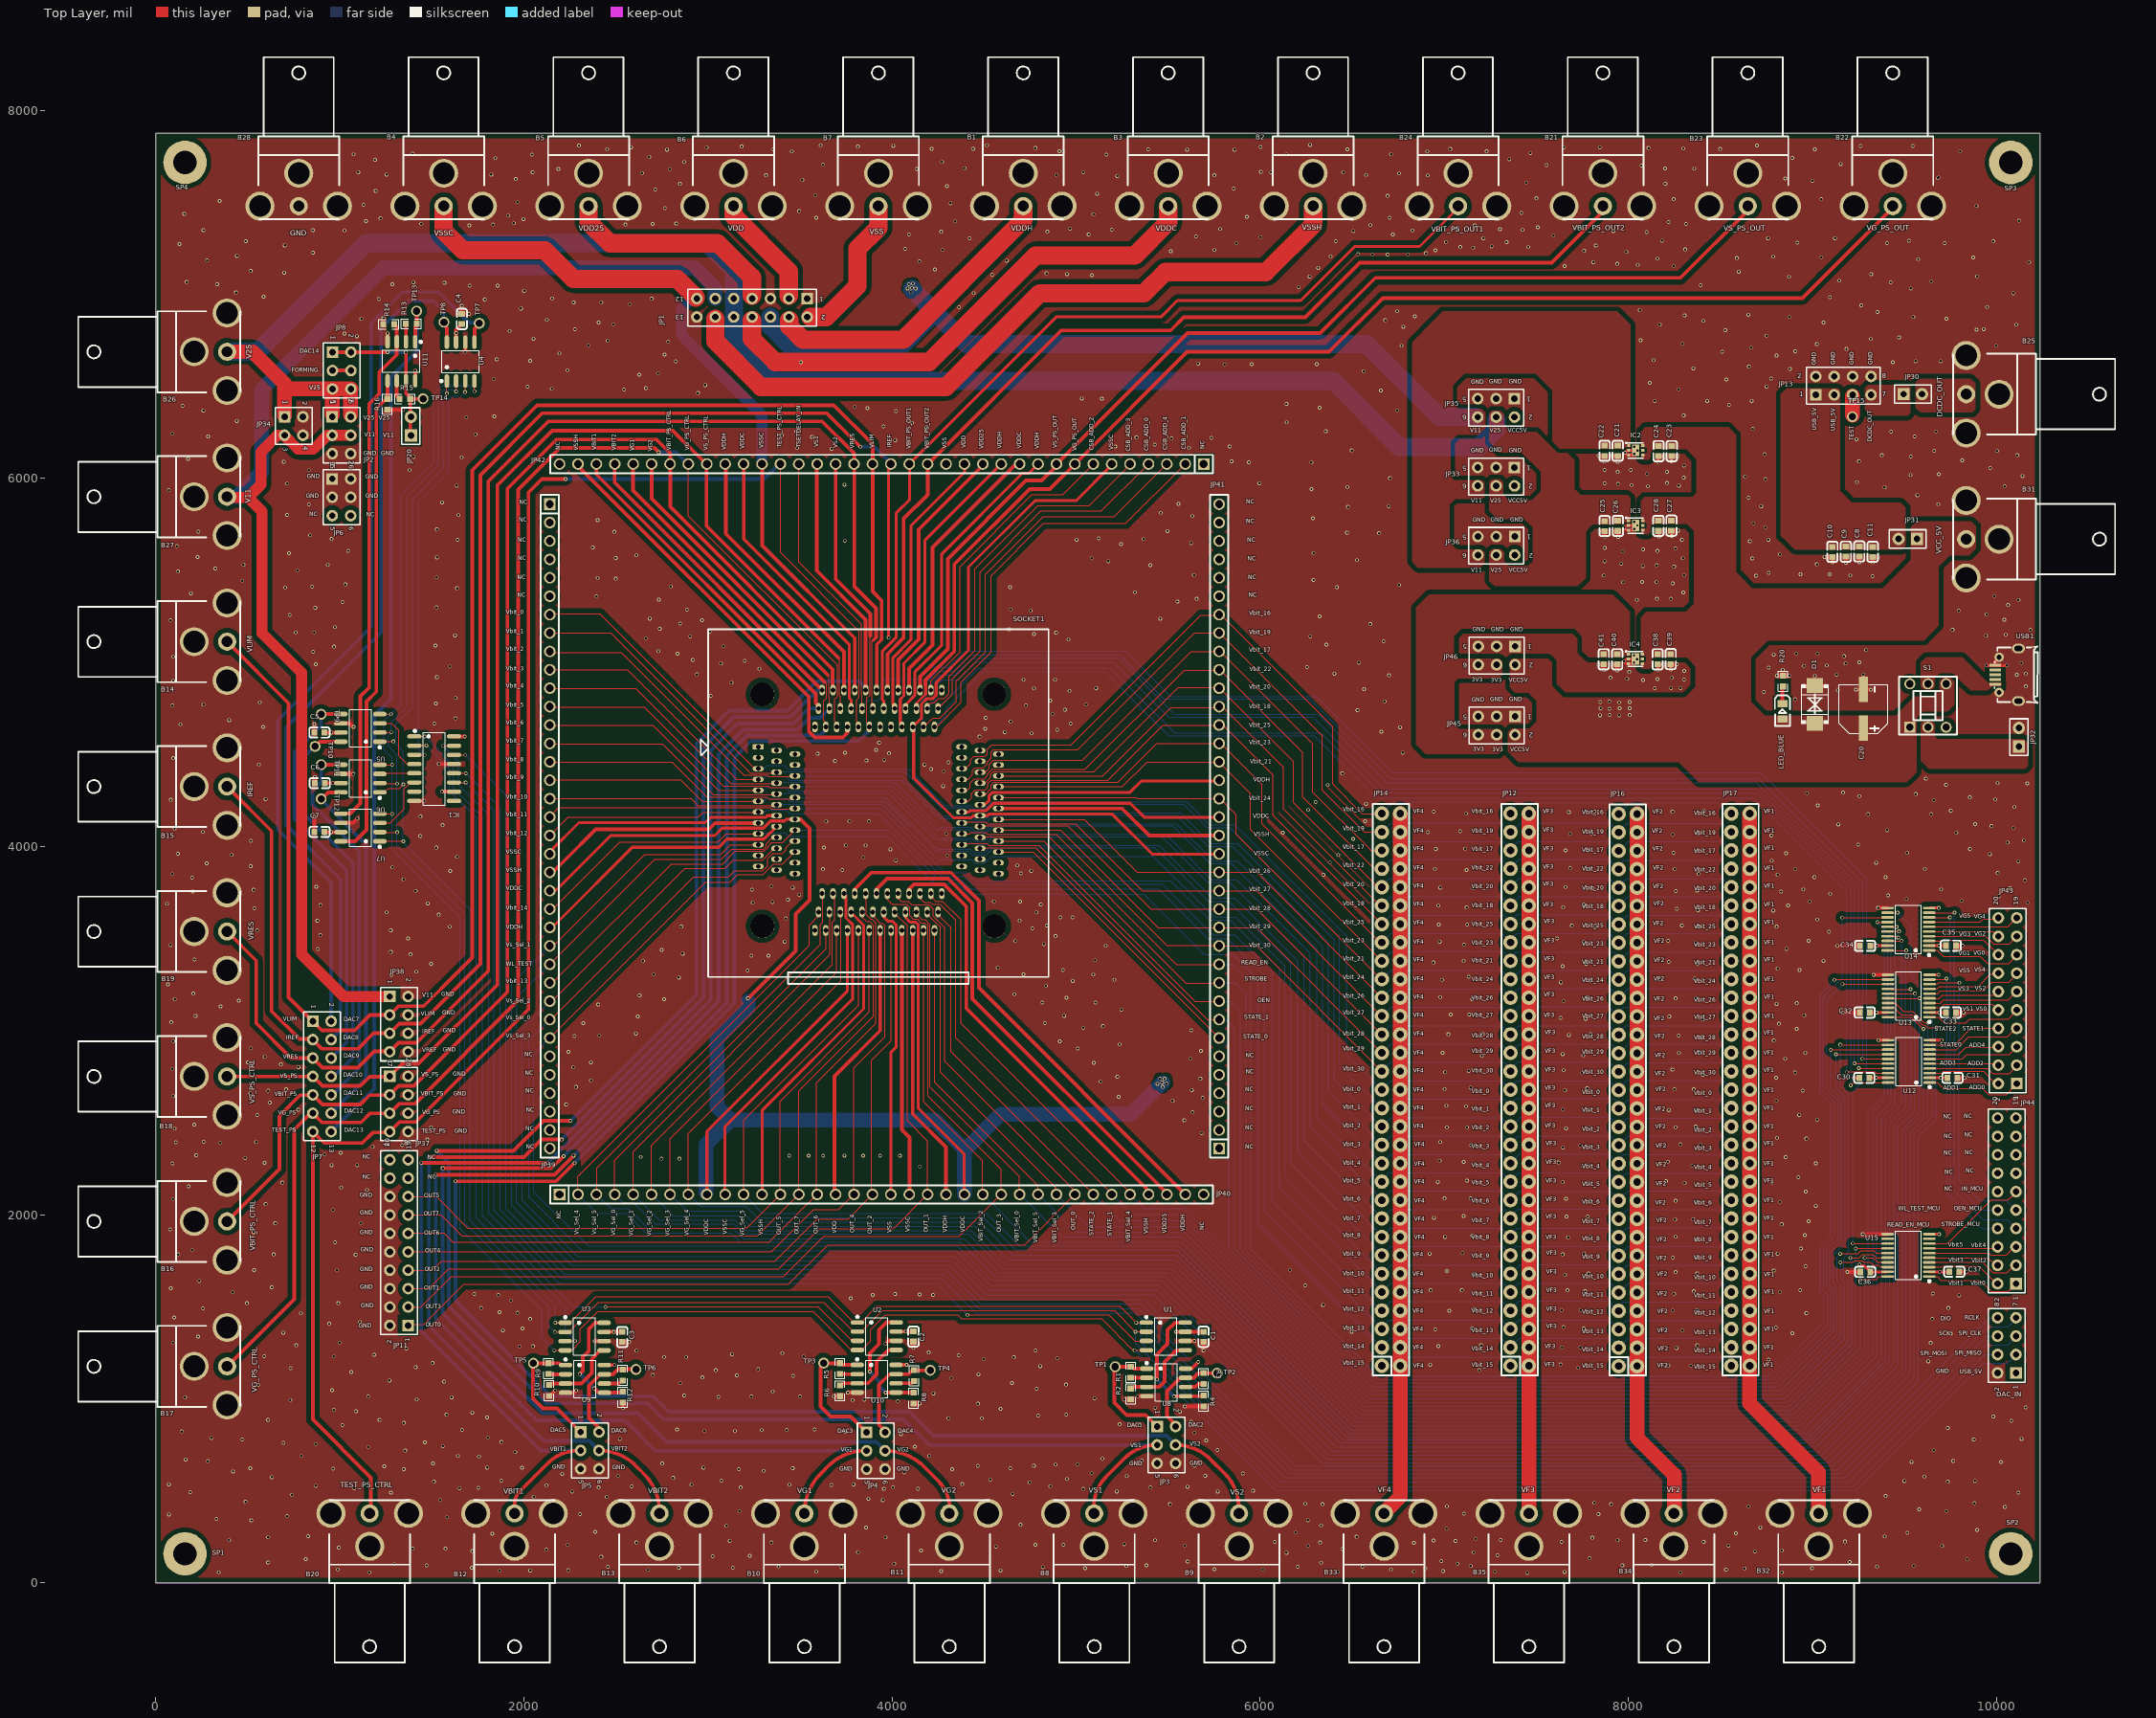
[diagram p0: Top Layer view]
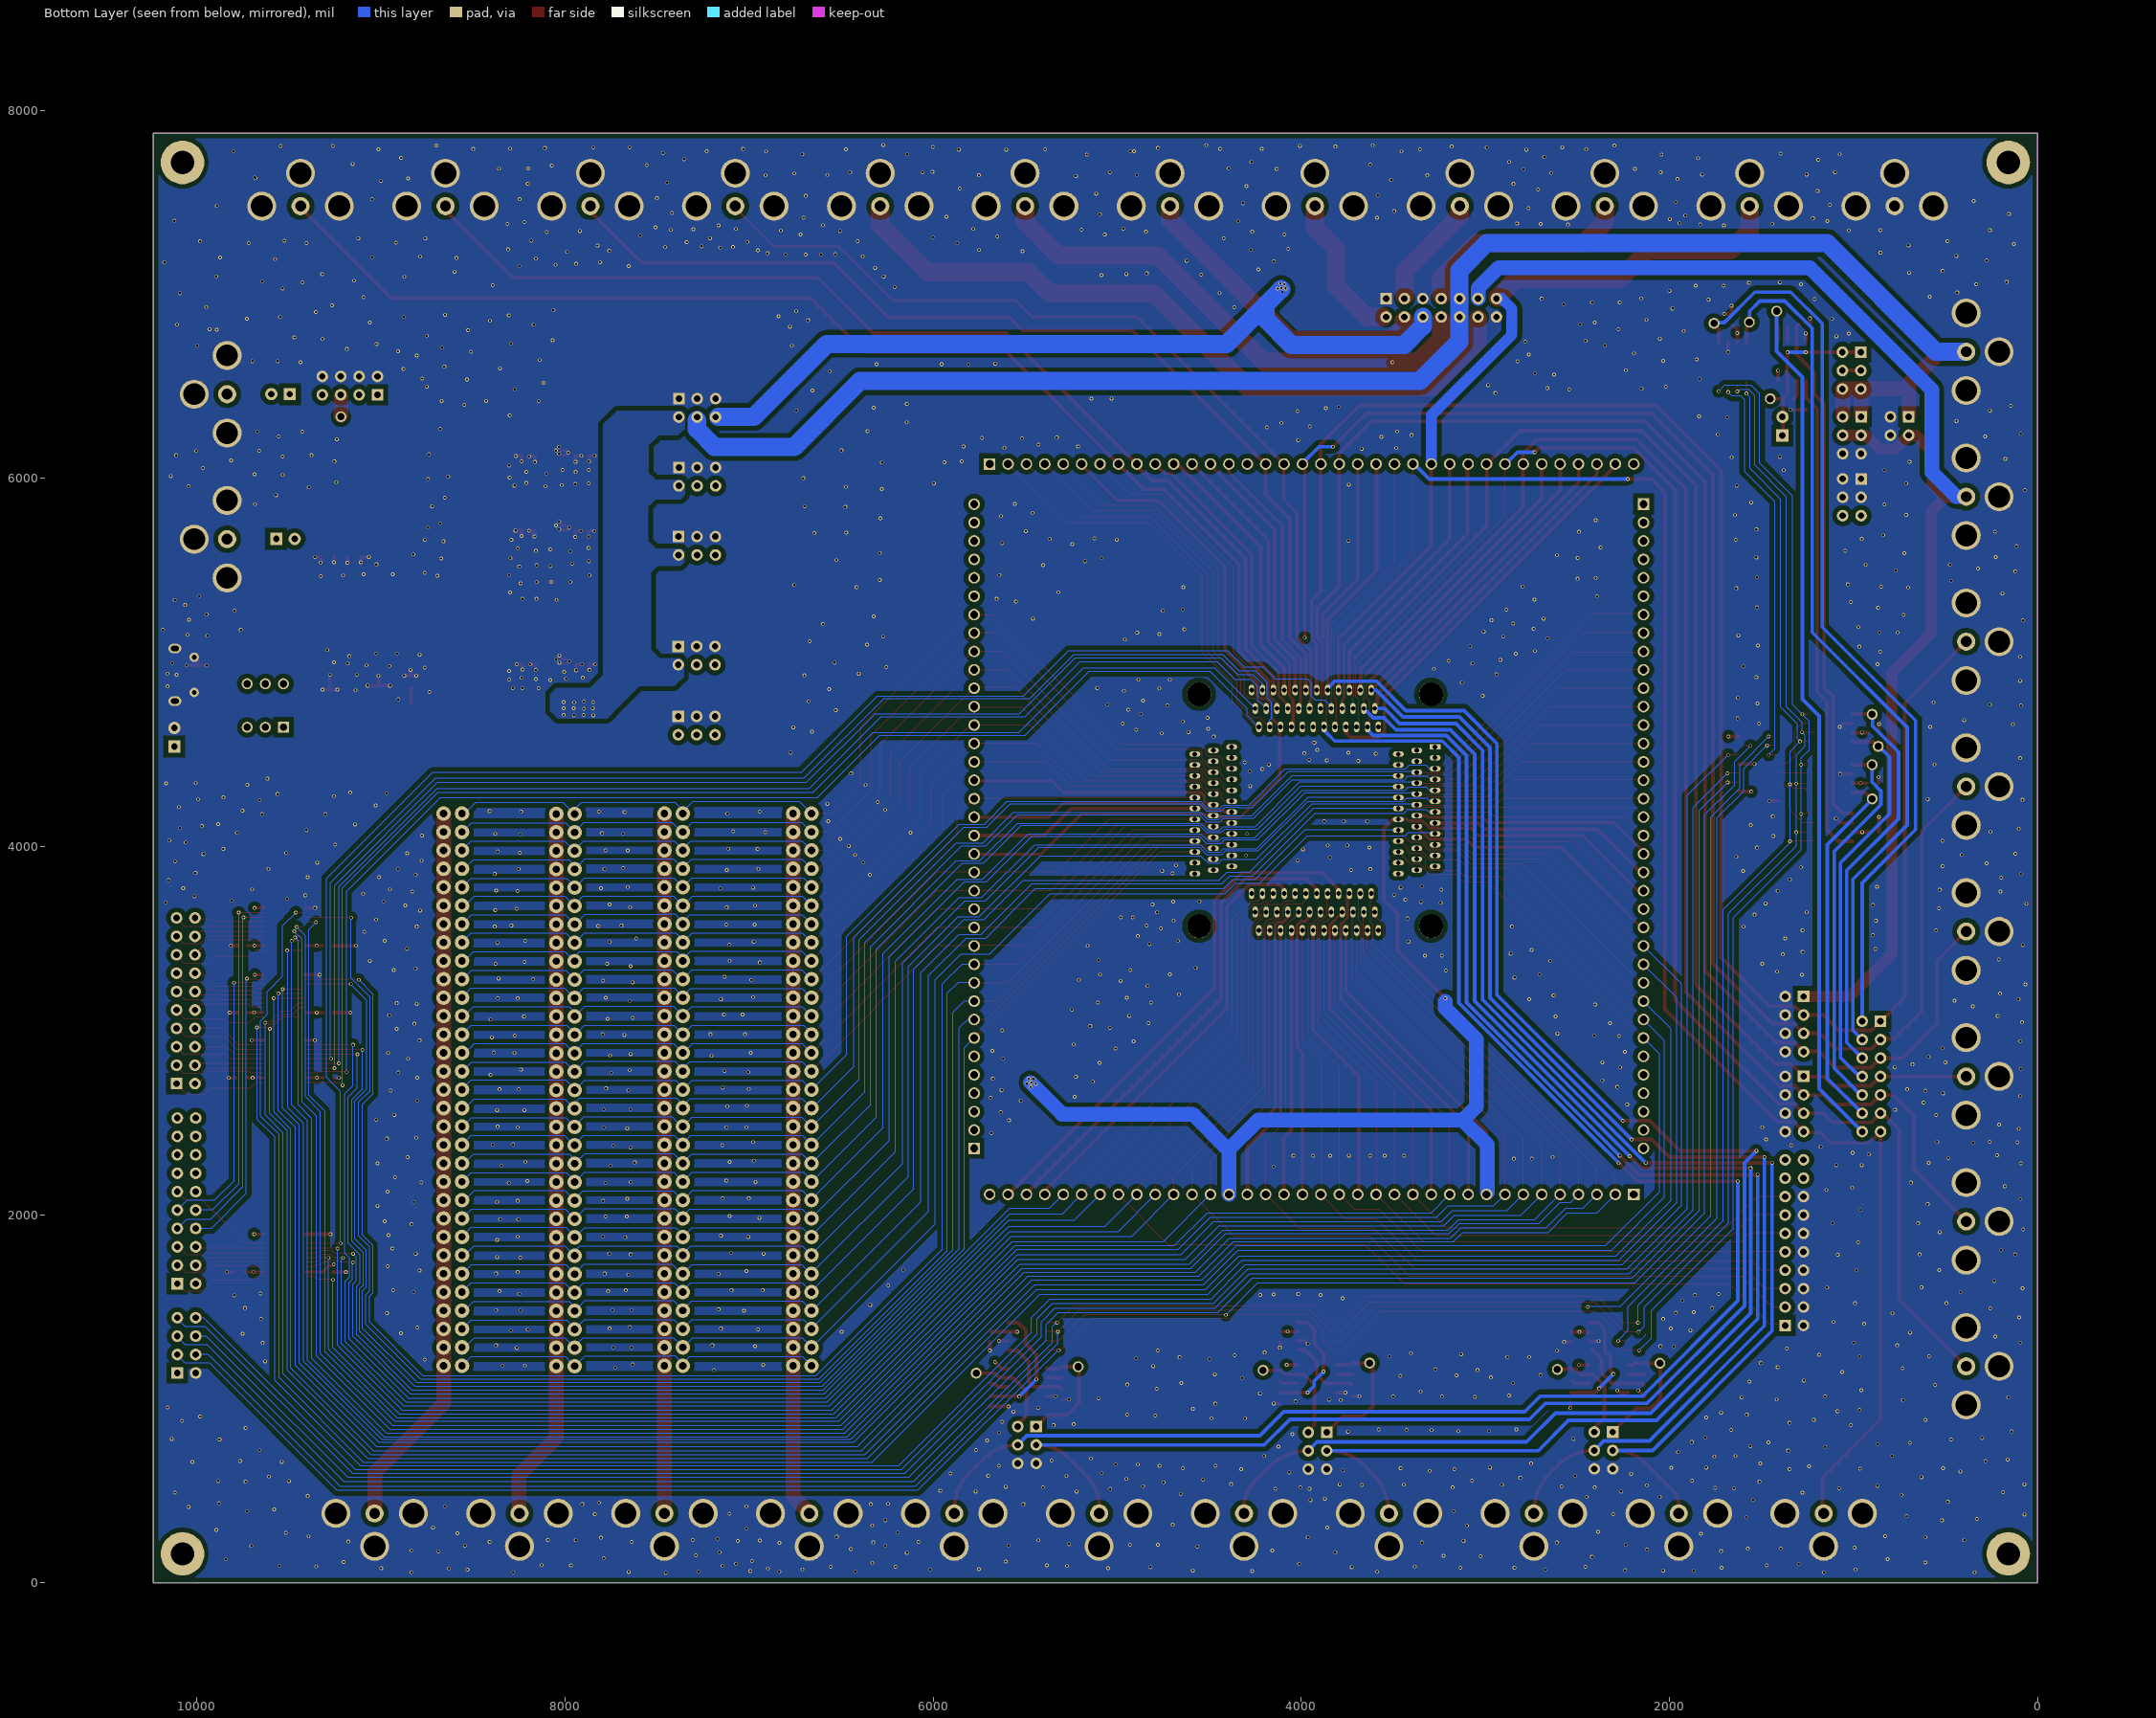
[diagram p1: Bottom Layer view, seen from below]
# Altium PCB MISC62794.PcbDoc (part 1 of 7)
Units mil, origin at the board's own origin, x right, y up, seen from the top; angles counter-clockwise.
Board outline 10236.22 x 7874.02 mil, 4 copper layers (Top Layer, GND, POWER, Bottom Layer); 158 components, 185 nets, 1211 pads, 1759 vias.

## Layer stack, top to bottom (the 12.6 mil dielectric is the usual default, probably not edited)
Top Layer: signal copper 1.4
Dielectric: core 12.6, FR-4, Dk 4.8
GND: plane copper 1.4, net GND
Dielectric: prepreg 12.6, FR-4, Dk 4.8
POWER: signal copper 1.4
Dielectric: core 12.6, FR-4, Dk 4.8
Bottom Layer: signal copper 1.4

## Board outline
0,0 10236.22,0 10236.22,7874.02 0,7874.02

## Design rules (kind name [scope] priority, off if disabled: settings)
Clearance Clearance_1 [inpolygon] p1: gap=6
Clearance [All] p2: gap=6
DiffPairsRouting [All] p1: maxlimit=10 minlimit=6 mostfreqgap=10 toplayer_maxgap=6 toplayer_prefgap=6 midlayer1_mingap=10 bottomlayer_maxgap=6 bottomlayer_prefgap=6 maxuncoupledlength=500
HoleSize [All] p1: absolutevalues=TRUE maxlimit=500 minlimit=1 maxpercent=80.000 minpercent=20.000
HoleToHoleClearance [All] p1: gap=0 allowstackedmicrovias=TRUE
MinimumSolderMaskSliver [All] p1: minsoldermaskwidth=0
PlaneClearance [All] p1: clearance=6
PlaneConnect [All] p1: planeconnectstyle=Direct reliefexpansion=20 reliefentries=4 reliefconductorwidth=10 reliefairgap=10
PolygonConnect [All] p1: connectstyle=Direct reliefconductorwidth=10 reliefentries=4 polygonreliefangle="90 Angle"
RoutingVias [All] p1: holewidth=12 width=20 viastyle="Through Hole" minholewidth=12 minwidth=20 maxholewidth=12 maxwidth=20
SilkToSilkClearance [All] p1: silktosilkclearance=0
SilkscreenOverComponentPads [All] p1: minsilkscreentomaskgap=0
SolderMaskExpansion [All] p1: expansion=4
Width [All] p1: maxlimit=200 minlimit=6 preferedwidth=10 toplayer_prefwidth=6 midlayer1_minwidth=10 bottomlayer_prefwidth=6 minimp=50.000000 maximp=50.000000 favimp=50.000000
20 further rules are at their usual default settings.

## Classes and differential pairs
component class PCB2: B1 B2 B3 B4 B5 B6 B7 B8 B9 B10 B11 B12 B13 B14 B15 B16 B17 B18 B19 B20 B21 B22 B23 B24 B25 B26 B27 B28 B32 B33 B34 B35 C20 C21 C22 C23 C24 C25 C26 C27 C28 C30 C31 C32 C33 C34 C35 C36 C37 C38 C39 C40 C41 D1 IC2 IC3 IC4 JP1 JP2 JP3 JP4 JP5 JP6 JP7 JP8 JP11 JP12 JP13 JP14 JP16 JP17 JP30 JP32 JP33 JP34 JP35 JP36 JP37 JP38 JP39 JP40 JP41 JP42 JP43 JP44 JP45 JP46 LED_BLUE R20 S1 SOCKET1 SP1 SP2 SP3 SP4 TP15 U12 U13 U14 U15 USB1
component class DacModule: B31 C1 C2 C3 C4 C5 C6 C7 C8 C9 C10 C11 DAC_IN IC1 JP20 JP31 R1 R2 R3 R4 R5 R6 R7 R8 R9 R10 R11 R12 R13 R14 R15 R16 TP1 TP2 TP3 TP4 TP5 TP6 TP7 TP8 TP9 TP10 TP11 TP12 TP13 TP14 U1 U2 U3 U4 U5 U6 U7 U8 U9 U10 U11

## Components (designator, comment, footprint, x,y, rotation, side; value= is the part's Value field where it differs from the comment)
B1 "bnc" BNC-TH_DOSIN-801-0072 4712.83,7658.31 r0 top
B2 "bnc" BNC-TH_DOSIN-801-0072 6287.64,7658.31 r0 top
B3 "bnc" BNC-TH_DOSIN-801-0072 5500.24,7658.31 r0 top
B4 "bnc" BNC-TH_DOSIN-801-0072 1563.23,7658.31 r0 top
B5 "bnc" BNC-TH_DOSIN-801-0072 2350.63,7658.31 r0 top
B6 "bnc" BNC-TH_DOSIN-801-0072 3138.03,7658.31 r0 top
B7 "bnc" BNC-TH_DOSIN-801-0072 3925.43,7658.31 r0 top
B8 "bnc" BNC-TH_DOSIN-801-0072 5098.01,198.02 r180 top
B9 "bnc" BNC-TH_DOSIN-801-0072 5885.41,198.02 r180 top
B10 "bnc" BNC-TH_DOSIN-801-0072 3523.2,198.02 r180 top
B11 "bnc" BNC-TH_DOSIN-801-0072 4310.61,198.02 r180 top
B12 "bnc" BNC-TH_DOSIN-801-0072 1948.4,198.02 r180 top
B13 "bnc" BNC-TH_DOSIN-801-0072 2735.8,198.02 r180 top
B14 "bnc" BNC-TH_DOSIN-801-0072 207.64,5113.09 r90 top
B15 "bnc" BNC-TH_DOSIN-801-0072 207.64,4325.69 r90 top
B16 "bnc" BNC-TH_DOSIN-801-0072 207.64,1963.49 r90 top
B17 "bnc" BNC-TH_DOSIN-801-0072 207.64,1176.09 r90 top
B18 "bnc" BNC-TH_DOSIN-801-0072 207.64,2750.89 r90 top
B19 "bnc" BNC-TH_DOSIN-801-0072 207.64,3538.29 r90 top
B20 "bnc" BNC-TH_DOSIN-801-0072 1161,198.02 r180 top
B21 "bnc" BNC-TH_DOSIN-801-0072 7862.44,7658.31 r0 top
B22 "bnc" BNC-TH_DOSIN-801-0072 9437.24,7658.31 r0 top
B23 "bnc" BNC-TH_DOSIN-801-0072 8649.84,7658.31 r0 top
B24 "bnc" BNC-TH_DOSIN-801-0072 7075.04,7658.31 r0 top
B25 "bnc" BNC-TH_DOSIN-801-0072 10015.29,6457.37 r270 top
B26 "bnc" BNC-TH_DOSIN-801-0072 207.64,6687.9 r90 top
B27 "bnc" BNC-TH_DOSIN-801-0072 207.64,5900.5 r90 top
B28 "bnc" BNC-TH_DOSIN-801-0072 775.83,7658.31 r0 top
B31 "bnc" BNC-TH_DOSIN-801-0072 10015.29,5669.97 r270 top
B32 "bnc" BNC-TH_DOSIN-801-0072 9035.02,198.02 r180 top
B33 "bnc" BNC-TH_DOSIN-801-0072 6672.81,198.02 r180 top
B34 "bnc" BNC-TH_DOSIN-801-0072 8247.61,198.02 r180 top
B35 "bnc" BNC-TH_DOSIN-801-0072 7460.21,198.02 r180 top
C1 "104" 0603C 5692.12,1336.67 r90 top
C2 "104" 0603C 4116.12,1337.67 r90 top
C3 "104" 0603C 2534.12,1335.67 r90 top
C4 "104" 0603C 1662,6866 r270 top
C5 "104" 0603C 888.54,4619.46 r0 top
C6 "104" 0603C 890.54,4344.46 r0 top
C7 "104" 0603C 888.54,4079.46 r0 top
C8 "104" 0603C 9255.29,5602.97 r270 top
C9 "104" 0603C 9182.29,5601.97 r270 top
C10 "104" 0603C 9109.29,5600.97 r270 top
C11 "104" 0603C 9328.29,5600.97 r270 top
C20 "100uF/25V" EC-D6.3x7.7 9278,4748 r90 top
C21 "100nF" 0603C 7942.56,6150.02 r270 top
C22 "10uF/16V" 0603C 7871.56,6150.02 r270 top
C23 "100nF" 0603C 8236.56,6148.02 r270 top
C24 "10uF/16V" 0603C 8164.56,6148.02 r270 top
C25 "100nF" 0603C 7871.56,5741.02 r270 top
C26 "10nF/16V" 0603C 7943.56,5742.02 r270 top
C27 "100nF" 0603C 8234.56,5743.02 r270 top
C28 "10nF/16V" 0603C 8163.56,5742.02 r270 top
C30 "100nF" 0603C 9283,2743.01 r0 top
C31 "100nF" 0603C 9762,2743.01 r0 top
C32 "100nF" 0603C 9285,3098.01 r0 top
C33 "100nF" 0603C 9753,3098.01 r0 top
C34 "100nF" 0603C 9287,3460.01 r0 top
C35 "100nF" 0603C 9753,3461.01 r0 top
C36 "100nF" 0603C 9288,1689.01 r0 top
C37 "100nF" 0603C 9772,1690.01 r0 top
C38 "10nF/16V" 0603C 8159.56,5017.02 r270 top
C39 "100nF" 0603C 8230.56,5018.02 r270 top
C40 "10nF/16V" 0603C 7939.56,5017.02 r270 top
C41 "100nF" 0603C 7866.56,5017.02 r270 top
D1 "SMBJ5.0CA" SMB 9014,4772 r90 top
DAC_IN "DAC_IN" HDR2.54-LI-2x4P 10057,1290 r90 top
IC1 "74HC595" SOIC-16_L9.9-W3.9-P1.27-LS6.0-BL 1511.64,4428.09 r270 top
IC2 "TPS74511PQWDRVRQ1" WSON-6_L2.0-W2.0-P0.65-BL-EP 8037.56,6152.02 r270 top
IC3 "TPS74525PQWDRVRQ1" WSON-6_L2.0-W2.0-P0.65-BL-EP 8036.56,5744.02 r270 top
IC4 "TPS74533PQWDRVRQ1" WSON-6_L2.0-W2.0-P0.65-BL-EP 8035.56,5019.02 r270 top
JP1 "HEADER 7X2" HDR2.54-LI-2x7P 3239,6927 r180 top
JP2 "HEADER 3X2" HDR2.54-LI-2x3P 1007.64,6234.52 r270 top
JP3 "HEADER 3X2" HDR2.54-LI-2x3P 5490.19,749.02 r270 top
JP4 "HEADER 3X2" HDR2.54-LI-2x3P 3911.48,717.38 r270 top
JP5 "HEADER 3X2" HDR2.54-LI-2x3P 2357.19,719.02 r270 top
JP6 "HEADER 2X2" HDR2.54-LI-2x3P 1007.64,5897.52 r270 top
JP7 "HEADER 7X2" HDR2.54-LI-2x7P 902,2751 r270 top
JP8 "HEADER 3X2" HDR2.54-LI-2x3P 1009,6586.02 r270 top
JP11 "HEADER 10X2" HDR2.54-LI-2x10P 1320.64,1848.09 r90 top
JP12 "HEADER 31X2" HDR2.54-LI-2x31P 7410,2679 r90 top locked
JP13 "HEADER 4X2" HDR2.54-LI-2x4P 9169,6504 r0 top
JP14 "HEADER 31X2" HDR2.54-LI-2x31P 6711,2679 r90 top
JP16 "HEADER 31X2" HDR2.54-LI-2x31P 7998,2677.02 r90 top locked
JP17 "HEADER 31X2" HDR2.54-LI-2x31P 8610,2679 r90 top locked
JP20 "HEADER 1X2" HDR2.54-LI-2P 1385,6284 r90 top
JP30 "HEADER 1X2" HDR2.54-LI-2P 9546,6458 r0 top
JP31 "HEADER 1X2" HDR2.54-LI-2P 9519.29,5670.97 r180 top
JP32 "HEADER 1X2" HDR2.54-LI-2P 10123,4594.02 r90 top
JP33 "HEADER 3X2" HDR2.54-LI-2x3P 7282,6009.46 r180 top
JP34 "HEADER 2X2" HDR2.54-LI-2x2P 748.64,6284.52 r270 top
JP35 "HEADER 3X2" HDR2.54-LI-2x3P 7282,6383.02 r180 top
JP36 "HEADER 3X2" HDR2.54-LI-2x3P 7283,5634 r180 top
JP37 "HEADER 4X2" HDR2.54-LI-2x4P 1319.93,2601.09 r270 top
JP38 "HEADER 4X2" HDR2.54-LI-2x4P 1319.93,3035.09 r270 top
JP39 "HEADER 36X1" HDR2.54-LI-1x36P 2140,4110.02 r270 top
JP40 "HEADER  36X1" HDR2.54-LI-1x36P 3943,2110.02 r0 top
JP41 "HEADER  36X1" HDR2.54-LI-1x36P 5777,4110.02 r90 top
JP42 "HEADER  36X1" HDR2.54-LI-1x36P 3943,6078.02 r180 top
JP43 "HEADER 10X2" HDR2.54-LI-2x10P 10061,3162.01 r90 top
JP44 "HEADER 10X2" HDR2.54-LI-2x10P 10057,2075.01 r90 top
JP45 "HEADER 3X2" HDR2.54-LI-2x3P 7285,4657 r180 top
JP46 "HEADER 3X2" HDR2.54-LI-2x3P 7285,5037.46 r180 top
LED_BLUE "LED" LED0805-R-RD 8838,4733.98 r270 top
R1 "1k" 0603R 5296.12,1143.67 r90 top
R2 "1k" 0603R 5296.12,1025.67 r270 top
R3 "1k" 0603R 5693.12,1109.67 r270 top
R4 "1k" 0603R 5693,988 r270 top
R5 "1k" 0603R 3717.12,1163.67 r90 top
R6 "1k" 0603R 3717.12,1043.67 r270 top
R7 "1k" 0603R 4119.12,1125.67 r270 top
R8 "1k" 0603R 4118,1004 r270 top
R9 "1k" 0603R 2134.12,1163.67 r90 top
R10 "1k" 0603R 2135.12,1044.67 r270 top
R11 "1k" 0603R 2535.12,1127.67 r270 top
R12 "1k" 0603R 2537,1008 r270 top
R13 "1k" 0603R 1387.29,6839.38 r0 top
R14 "1k" 0603R 1265.29,6838.38 r180 top
R15 "1k" 0603R 1352.29,6432.38 r180 top
R16 "1k" 0603R 1258.29,6402.38 r270 top
R20 "1k" 0603R 8840,4899 r90 top
S1 "TK-6700-1" SW-TH_6P-L8.0-W8.0-P2.50 9628.73,4765.88 r0 top
SOCKET1 "M189" YAMAICHI_IC51-1444-1354-7 3925,4197.02 r0 top locked
SP1 "M3" M3 157.48,157.48 r0 top locked
SP2 "M3" M3 10078.74,157.48 r0 top locked
SP3 "M3" M3 10078.74,7716.54 r0 top locked
SP4 "M3" M3 157.48,7716.54 r0 top locked
TP1 "OUT1" TP1.0 5212.12,1173.67 r0 top
TP2 "OUT2" TP1.0 5766.12,1138.67 r90 top
TP3 "OUT3" TP1.0 3628.12,1193.67 r90 top
TP4 "OUT4" TP1.0 4207.12,1154.67 r90 top
TP5 "OUT5" TP1.0 2051.12,1192.67 r90 top
TP6 "OUT6" TP1.0 2608,1159 r90 top
TP7 "OUT7" TP1.0 1756.71,6842.62 r180 top
TP8 "OUT8" TP1.0 1565,6849 r180 top
TP9 "OUT9" TP1.0 897.54,4718.46 r0 top
TP10 "OUT10" TP1.0 864.54,4544.46 r0 top
TP11 "OUT11" TP1.0 897.54,4444.46 r0 top
TP12 "OUT12" TP1.0 897.24,4259.09 r0 top
TP13 "OUT13" TP1.0 1416,6909 r0 top
TP14 "OUT14" TP1.0 1451,6433 r0 top
TP15 "3V3" TP1.0 9218,6335 r90 top
U1 "LTC1446" SO-8 5487.12,1338.67 r0 top
U2 "LTC1446" SO-8 3917.12,1339.67 r0 top
U3 "LTC1446" SO-8 2329.12,1337.67 r0 top
U4 "LTC1446" SO-8 1655.71,6634.62 r90 top
U5 "LTC1446" SO-8 1110.54,4644.46 r180 top
U6 "LTC1446" SO-8 1110.54,4369.46 r180 top
U7 "LTC1446" SO-8 1110.54,4103.46 r180 top
U8 "LM358" SO-8 5489.12,1088.67 r0 top
U9 "LM358" SO-8 2331.12,1107.67 r0 top
U10 "LM358" SO-8 3916.12,1108.67 r0 top
U11 "LM358" SO-8 1333.29,6636.38 r270 top
U12 "TXS0108E" TSSOP-20_L6.5-W4.4-P0.65-LS6.4-BL 9525,2833.01 r180 top
U13 "TXS0108E" TSSOP-20_L6.5-W4.4-P0.65-LS6.4-BL 9524,3188.01 r180 top
U14 "TXS0108E" TSSOP-20_L6.5-W4.4-P0.65-LS6.4-BL 9522,3551.01 r180 top
U15 "TXS0108E" TSSOP-20_L6.5-W4.4-P0.65-LS6.4-BL 9523,1779.01 r180 top
USB1 "MICROXNJ" MICRO-USB-SMD_MICROXNJ 10097.73,4932.88 r90 top

## Footprints (in the part's own frame and the unit in brackets; to place one, negate y for a bottom-side part, rotate by r counter-clockwise, add the part's x,y. Pads: shape width x height; smd on the part's side, far side on the other; paste and mask are expansions set on the pad)
0603C [mm]
  rect 0.8x0.9 smd: 1(-0.7,0) 2(0.7,0)
  silkscreen extent -1.41,-0.71 1.39,0.72
0603R [mil]
  rect 31.75x34.02 smd paste-3937.01 mask+2: 1(-29.66,0) 2(29.66,0)
  silkscreen extent -55,-26 55,26
BNC-TH_DOSIN-801-0072 [mm]
  round 2.5 hole 1.5 paste+0 mask+0.051: 1(0,-4.55)
  round 4 hole 3 paste+0 mask+0.051: 2(5.35,-4.55) 3(-5.35,-4.55) 4(0,0)
  silkscreen extent -5.59,-6.35 5.59,16
EC-D6.3x7.7 [mm]
  rect 3.5x1.2 smd: 1(-2.67,0) 2(2.67,0)
  silkscreen extent -3.38,-3.38 3.38,3.38
HDR2.54-LI-1x36P [mm]
  rect 1.6x1.6 hole 1.1: 1(-44.45,0)
  round 1.6 hole 1.1: 2(-41.91,0) 3(-39.37,0) 4(-36.83,0) 5(-34.29,0) 6(-31.75,0) 7(-29.21,0) 8(-26.67,0) 9(-24.13,0) 10(-21.59,0) 11(-19.05,0) 12(-16.51,0) 13(-13.97,0) 14(-11.43,0) 15(-8.89,0) 16(-6.35,0) 17(-3.81,0) 18(-1.27,0) 19(1.27,0) 20(3.81,0) 21(6.35,0) 22(8.89,0) 23(11.43,0) 24(13.97,0) 25(16.51,0) 26(19.05,0) 27(21.59,0) 28(24.13,0) 29(26.67,0) 30(29.21,0) 31(31.75,0) 32(34.29,0) 33(36.83,0) 34(39.37,0) 35(41.91,0) 36(44.45,0)
  silkscreen extent -45.72,-1.27 45.72,1.27
HDR2.54-LI-2P [mm] "排针，2脚"
  rect 1.7x1.7 hole 0.9: 1(-1.27,0)
  round 1.7 hole 0.9: 2(1.27,0)
  silkscreen extent -2.54,-1.27 2.54,1.27, body extent -2.54,-1.27 2.54,1.27, height 2.54
HDR2.54-LI-2x2P [mm]
  rect 1.6x1.6 hole 0.9: 1(-1.27,-1.27)
  round 1.6 hole 0.9: 2(-1.27,1.27) 3(1.27,-1.27) 4(1.27,1.27)
  silkscreen extent -2.54,-2.54 2.54,2.54, body extent -2.54,-2.54 2.54,2.54, height 8.5
HDR2.54-LI-2x3P [mm] "双排排针，2x3脚"
  rect 1.6x1.6 hole 0.9: 1(-2.54,-1.27)
  round 1.6 hole 0.9: 2(-2.54,1.27) 3(0,-1.27) 4(0,1.27) 5(2.54,-1.27) 6(2.54,1.27)
  silkscreen extent -3.81,-2.54 3.81,2.54, body extent -3.81,-2.54 3.81,2.54, height 8.5
HDR2.54-LI-2x4P [mm] "双排排针，4x2脚"
  rect 1.6x1.6 hole 0.9: 1(-3.81,-1.27)
  round 1.6 hole 0.9: 2(-3.81,1.27) 3(-1.27,-1.27) 4(-1.27,1.27) 5(1.27,-1.27) 6(1.27,1.27) 7(3.81,-1.27) 8(3.81,1.27)
  silkscreen extent -5.08,-2.54 5.08,2.54, body extent -5.08,-2.54 5.08,2.54, height 8.5
HDR2.54-LI-2x7P [mm] "双排排针，7x2脚"
  rect 1.6x1.6 hole 0.9: 1(-7.62,-1.27)
  round 1.6 hole 0.9: 2(-7.62,1.27) 3(-5.08,-1.27) 4(-5.08,1.27) 5(-2.54,-1.27) 6(-2.54,1.27) 7(0,-1.27) 8(0,1.27) 9(2.54,-1.27) 10(2.54,1.27) 11(5.08,-1.27) 12(5.08,1.27) 13(7.62,-1.27) 14(7.62,1.27)
  silkscreen extent -8.89,-2.54 8.89,2.54, body extent -8.89,-2.54 8.89,2.54, height 8.5